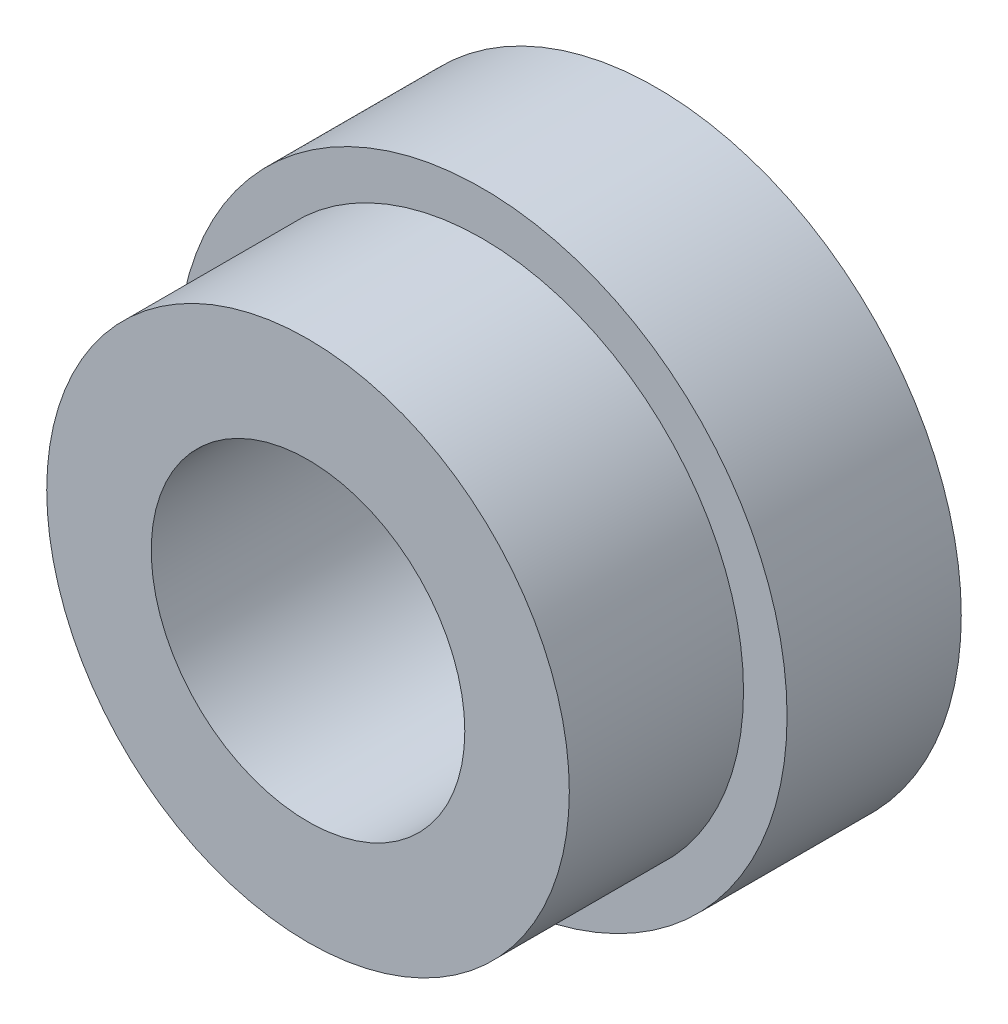
SolidWorks part; units mm, degrees
ref_plane "Front Plane" through (0, 0, 0) normal (0, 0, 1) x (1, 0, 0)
ref_plane "Top Plane" through (0, 0, 0) normal (0, 1, 0) x (1, 0, 0)
ref_plane "Right Plane" through (0, 0, 0) normal (1, 0, 0) x (0, 0, -1)
sketch "Sketch1" plane through (0, 0, 0) normal (0, 0, 1) x (1, 0, 0)
  circle A0 centre (0, 0) radius 17.5
extrude "Boss-Extrude1" add sketch "Sketch1" along normal blind 10
sketch "Sketch3" plane through (0, 0, 10) normal (0, 0, 1) x (1, 0, 0)
  circle A0 centre (0, 0) radius 15
extrude "Boss-Extrude2" add sketch "Sketch3" along normal blind 10
sketch "Sketch4" plane through (0, 0, 20) normal (0, 0, 1) x (1, 0, 0)
  circle A0 centre (0, 0) radius 9
extrude "Cut-Extrude1" cut sketch "Sketch4" against normal through all
